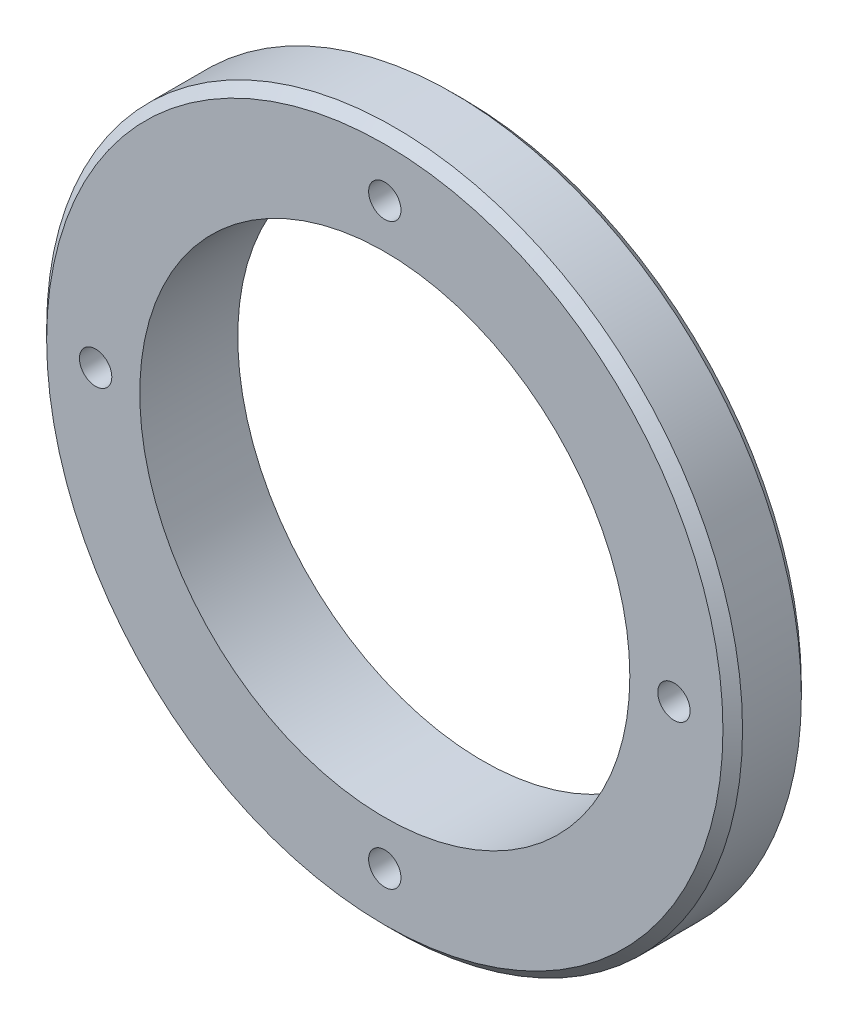
SolidWorks part; units mm, degrees
material "Q235B"
ref_plane "Front Plane" through (0, 0, 0) normal (0, 0, 1) x (1, 0, 0)
ref_plane "Top Plane" through (0, 0, 0) normal (0, 1, 0) x (1, 0, 0)
ref_plane "Right Plane" through (0, 0, 0) normal (1, 0, 0) x (0, 0, -1)
sketch "Sketch1" plane through (0, 0, 0) normal (0, 0, 1) x (1, 0, 0)
  circle A0 centre (0, 0) radius 35.5
  circle A1 centre (0, 0) radius 25
  dimension "D1" = 71
  dimension "D2" = 50
extrude "Boss-Extrude1" add sketch "Sketch1" along normal blind 10
sketch "Sketch2" plane through (0, 0, 10) normal (0, 0, 1) x (1, 0, 0)
  circle A0 centre (0, 0) radius 29.5 construction
  circle A1 centre (0, 29.5) radius 1.25
  circle A2 centre (29.5, 0) radius 1.25
  circle A3 centre (0, -29.5) radius 1.25
  circle A4 centre (-29.5, 0) radius 1.25
  dimension "D1" = 59
  dimension "D2" = 2.5
  dimension "D3" = 4
extrude "Cut-Extrude1" cut sketch "Sketch2" against normal through all
sketch "Sketch3" plane through (0, 0, 0) normal (0, 0, -1) x (-1, 0, 0)
  circle A0 centre (0, 0) radius 35.5
  circle A1 centre (0, 0) radius 26.5
  circle A2 centre (0, 0) radius 35.5 construction
  dimension "D1" = 53
extrude "Cut-Extrude2" cut sketch "Sketch3" against normal blind 2
hole_wizard "M4 Tapped Hole1" positions "Sketch4" profile "Sketch5" tap size "M4" standard "GB" end condition through all
sketch "Sketch4" plane through (0, 0, 10) normal (0, 0, 1) x (1, 0, 0)
  point P0 (0, -29.5)
  point P3 (-29.5, 0)
  point P6 (0, 29.5)
  point P9 (29.5, 0)
sketch "Sketch5" plane through (0, -29.5, 10) normal (1, 0, 0) x (0, -1, 0)
  line L0 (0, 0) -> (0, 10)
  line L1 (0, 10) -> (1.65, 10)
  line L2 (1.65, 10) -> (1.65, 0)
  line L5 (1.65, 0) -> (0, 0)
  line L11 (0, -6.35) -> (0, 107.95) construction
  dimension "通孔螺纹孔钻头直径" = 3.3
  dimension "通孔螺纹孔钻头深度" = 10
cosmetic thread "Cosmetic-Thread1" parameters "D2"=4
cosmetic thread "Cosmetic-Thread2" parameters "D2"=4
cosmetic thread "Cosmetic-Thread3" parameters "D2"=4
cosmetic thread "Cosmetic-Thread4" parameters "D2"=4
chamfer "Chamfer1" distance 1 angle 45 2 edges at (-35.5, 0, 2) (35.5, 0, 10)
